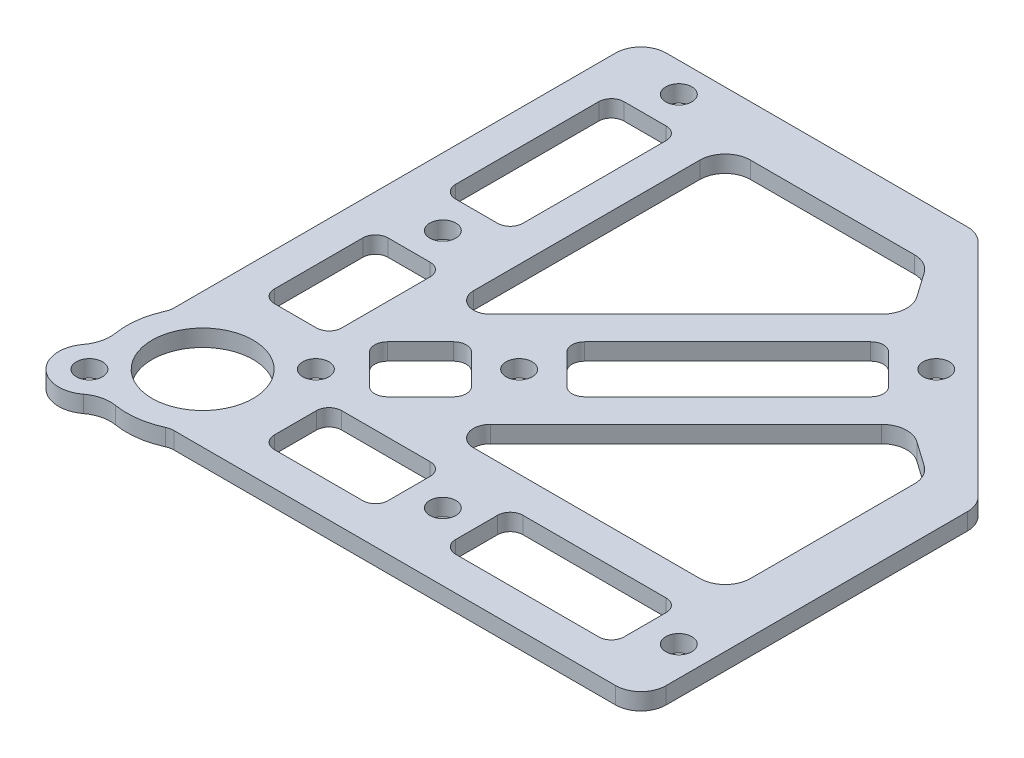
from build123d import *

# Parameters (mm, degrees)
SKETCH_1_R      = 6
SKETCH_1_R_2    = 1.55
SKETCH_1_W      = 13.5
SKETCH_1_H      = 8
SKETCH_1_W_2    = 8
SKETCH_1_H_2    = 13.5
SKETCH_1_W_3    = 20
SKETCH_1_H_3    = 20
EXTRUDE_1_DEPTH = 2
FILLET_1_R      = 2
FILLET_2_R      = 1.5
FILLET_3_R      = 3
FILLET_4_R      = 4


with BuildPart() as part:
    # 草图1 → 凸台-拉伸1 (new body)
    with BuildSketch(Plane(origin=(0, 0, 0), x_dir=(1, 0, 0), z_dir=(0, 1, 0))):
        with BuildLine():
            Line((4.123105626, -8), (60, -8))
            Line((60, -8), (60, 32))
            Line((60, 32), (32, 60))
            Line((32, 60), (-8, 60))
            Line((-8, 60), (-8, 4.123105626))
            ThreePointArc((-8, 4.123105626), (-8.992056265, 0.378053083), (-8.317851846, -3.437054068))
            ThreePointArc((-8.317851846, -3.437054068), (-9.298454173, -9.298454173), (-3.437054068, -8.317851846))
            ThreePointArc((-3.437054068, -8.317851846), (0.378053083, -8.992056265), (4.123105626, -8))
        make_face()
        with Locations(Location((0, 0, 0), (0, 0, 270))):
            Circle(SKETCH_1_R, mode=Mode.SUBTRACT)
        with Locations(Location((6.717514421, 6.717514421, 0), (0, 0, 270))):
            Circle(SKETCH_1_R_2, mode=Mode.SUBTRACT)
        with Locations((17.75, 0)):
            Rectangle(SKETCH_1_W, SKETCH_1_H, mode=Mode.SUBTRACT)
        with Locations((0, 17.75)):
            Rectangle(SKETCH_1_W_2, SKETCH_1_H_2, mode=Mode.SUBTRACT)
        Polygon((12.727922061, 7.071067812), (7.071067812, 12.727922061), (13.119534675, 18.776388924), (18.776388924, 13.119534675), align=None, mode=Mode.SUBTRACT)
        with Locations(Location((18.776388924, 18.776388924, 0), (0, 0, 270))):
            Circle(SKETCH_1_R_2, mode=Mode.SUBTRACT)
        with Locations(Location((28.5, 0, 0), (0, 0, 270))):
            Circle(SKETCH_1_R_2, mode=Mode.SUBTRACT)
        with Locations((42.5, 0)):
            Rectangle(SKETCH_1_W_3, SKETCH_1_H, mode=Mode.SUBTRACT)
        with Locations(Location((56.5, 0, 0), (0, 0, 270))):
            Circle(SKETCH_1_R_2, mode=Mode.SUBTRACT)
        Polygon((54, 8), (19.313708499, 8), (47.714713492, 36.401004993), (54, 32), align=None, mode=Mode.SUBTRACT)
        with Locations(Location((0, 28.5, 0), (0, 0, 270))):
            Circle(SKETCH_1_R_2, mode=Mode.SUBTRACT)
        Polygon((36.401004993, 47.714713492), (8, 19.313708499), (8, 54), (32, 54), align=None, mode=Mode.SUBTRACT)
        with Locations((0, 42.5)):
            Rectangle(SKETCH_1_W_2, SKETCH_1_H_3, mode=Mode.SUBTRACT)
        with Locations(Location((0, 56.5, 0), (0, 0, 270))):
            Circle(SKETCH_1_R_2, mode=Mode.SUBTRACT)
        Polygon((24.433243174, 18.776388924), (18.776388924, 24.433243174), (37.868272016, 43.525126266), (43.525126266, 37.868272016), align=None, mode=Mode.SUBTRACT)
        with Locations(Location((43.525126266, 43.525126266, 0), (0, 0, 270))):
            Circle(SKETCH_1_R_2, mode=Mode.SUBTRACT)
        with Locations(Location((-6.717514421, -6.717514421, 0), (0, 0, 270))):
            Circle(SKETCH_1_R_2, mode=Mode.SUBTRACT)
    extrude(amount=EXTRUDE_1_DEPTH)

    # 圆角1
    fillet_1_edges = [part.edges().sort_by_distance(p)[0] for p in [
        (19.313708499, 1, -8),
        (8, 1, -19.313708499),
        (-8, 1, -4.123105626),
        (4.123105626, 1, 8),
    ]]
    fillet(fillet_1_edges, radius=FILLET_1_R)

    # 圆角2
    fillet_2_edges = [part.edges().sort_by_distance(p)[0] for p in [
        (7.071067812, 1, -12.727922061),
        (12.727922061, 1, -7.071067812),
        (18.776388924, 1, -13.119534675),
        (13.119534675, 1, -18.776388924),
        (18.776388924, 1, -24.433243174),
        (24.433243174, 1, -18.776388924),
        (43.525126266, 1, -37.868272016),
        (37.868272016, 1, -43.525126266),
        (32.5, 1, -4),
        (32.5, 1, 4),
        (52.5, 1, 4),
        (52.5, 1, -4),
        (11, 1, -4),
        (11, 1, 4),
        (24.5, 1, 4),
        (24.5, 1, -4),
        (4, 1, -52.5),
        (-4, 1, -52.5),
        (-4, 1, -32.5),
        (4, 1, -32.5),
        (4, 1, -11),
        (4, 1, -24.5),
        (-4, 1, -24.5),
        (-4, 1, -11),
    ]]
    fillet(fillet_2_edges, radius=FILLET_2_R)

    # 圆角3
    fillet_3_edges = [part.edges().sort_by_distance(p)[0] for p in [
        (54, 1, -8),
        (54, 1, -32),
        (47.714713492, 1, -36.401004993),
        (36.401004993, 1, -47.714713492),
        (32, 1, -54),
        (8, 1, -54),
        (-8, 1, -60),
        (32, 1, -60),
        (60, 1, -32),
        (60, 1, 8),
    ]]
    fillet(fillet_3_edges, radius=FILLET_3_R)

    # 圆角4
    fillet_4_edges = [part.edges().sort_by_distance(p)[0] for p in [
        (-8.317851846, 1, 3.437054068),
        (-3.437054068, 1, 8.317851846),
    ]]
    fillet(fillet_4_edges, radius=FILLET_4_R)


solid = part.part
